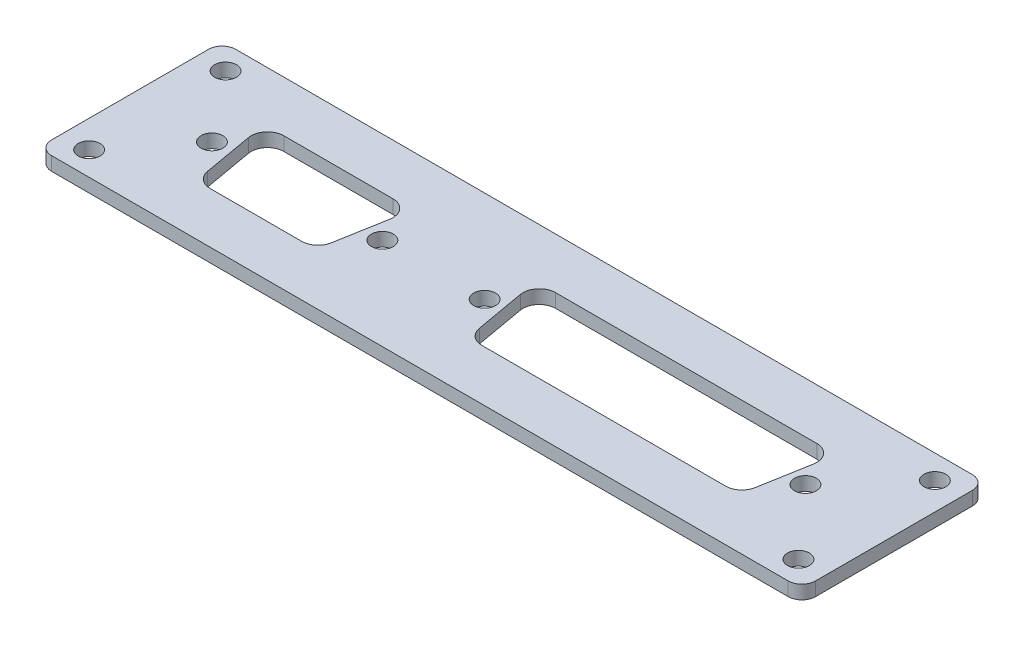
from build123d import *

# Parameters (mm, degrees)
SKETCH1_W           = 112
SKETCH1_H           = 27
BOSS_EXTRUDE1_DEPTH = 2
SKETCH2_R           = 1.6
CUT_EXTRUDE1_DEPTH  = 58.638962517
FILLET1_R           = 2
SKETCH3_R           = 1.6
CUT_EXTRUDE2_DEPTH  = 2


with BuildPart() as part:
    # Sketch1 → Boss-Extrude1 (new body)
    with BuildSketch(Plane(origin=(0, 0, 0), x_dir=(1, 0, 0), z_dir=(0, 1, 0))):
        Rectangle(SKETCH1_W, SKETCH1_H)
    extrude(amount=BOSS_EXTRUDE1_DEPTH)

    # Sketch2 → Cut-Extrude1 (cut, through all)
    with BuildSketch(Plane(origin=(0, 2, 0), x_dir=(1, 0, 0), z_dir=(0, 1, 0))):
        with Locations(Location((-52, 10, 0), (0, 0, 270))):
            Circle(SKETCH2_R)
        with Locations(Location((52, 10, 0), (0, 0, 270))):
            Circle(SKETCH2_R)
        with Locations(Location((52, -10, 0), (0, 0, 270))):
            Circle(SKETCH2_R)
        with Locations(Location((-52, -10, 0), (0, 0, 270))):
            Circle(SKETCH2_R)
    extrude(amount=-CUT_EXTRUDE1_DEPTH, mode=Mode.SUBTRACT)

    # Fillet1
    fillet1_edges = [part.edges().sort_by_distance(p)[0] for p in [
        (56, 1, 13.5),
        (-56, 1, 13.5),
        (-56, 1, -13.5),
        (56, 1, -13.5),
    ]]
    fillet(fillet1_edges, radius=FILLET1_R)

    # Sketch3 → Cut-Extrude2 (cut)
    with BuildSketch(Plane(origin=(0, 2, 0), x_dir=(1, 0, 0), z_dir=(0, 1, 0))):
        with BuildLine():
            Line((1.637186959, -6.05), (37.362813041, -6.05))
            ThreePointArc((37.362813041, -6.05), (38.905503304, -5.488506663), (39.726351648, -4.066755626))
            Line((39.726351648, -4.066755626), (41.013538607, 3.233244374))
            ThreePointArc((41.013538607, 3.233244374), (40.488506663, 5.192690263), (38.65, 6.05))
            Line((38.65, 6.05), (0.35, 6.05))
            ThreePointArc((0.35, 6.05), (-1.488506663, 5.192690263), (-2.013538607, 3.233244374))
            Line((-2.013538607, 3.233244374), (-0.726351648, -4.066755626))
            ThreePointArc((-0.726351648, -4.066755626), (0.094496696, -5.488506663), (1.637186959, -6.05))
        make_face()
        with BuildLine():
            Line((-23.5, 6.05), (-39.5, 6.05))
            ThreePointArc((-39.5, 6.05), (-41.338506663, 5.192690263), (-41.863538607, 3.233244374))
            Line((-41.863538607, 3.233244374), (-40.576351648, -4.066755626))
            ThreePointArc((-40.576351648, -4.066755626), (-39.755503304, -5.488506663), (-38.212813041, -6.05))
            Line((-38.212813041, -6.05), (-24.787186959, -6.05))
            ThreePointArc((-24.787186959, -6.05), (-23.244496696, -5.488506663), (-22.423648352, -4.066755626))
            Line((-22.423648352, -4.066755626), (-21.136461393, 3.233244374))
            ThreePointArc((-21.136461393, 3.233244374), (-21.661493337, 5.192690263), (-23.5, 6.05))
        make_face()
        with Locations(Location((-43.995, 0, 0), (0, 0, 270))):
            Circle(SKETCH3_R)
        with Locations(Location((-19.005, 0, 0), (0, 0, 270))):
            Circle(SKETCH3_R)
        with Locations(Location((-4.02, 0, 0), (0, 0, 270))):
            Circle(SKETCH3_R)
        with Locations(Location((43.02, 0, 0), (0, 0, 270))):
            Circle(SKETCH3_R)
    extrude(amount=-CUT_EXTRUDE2_DEPTH, mode=Mode.SUBTRACT)


solid = part.part
